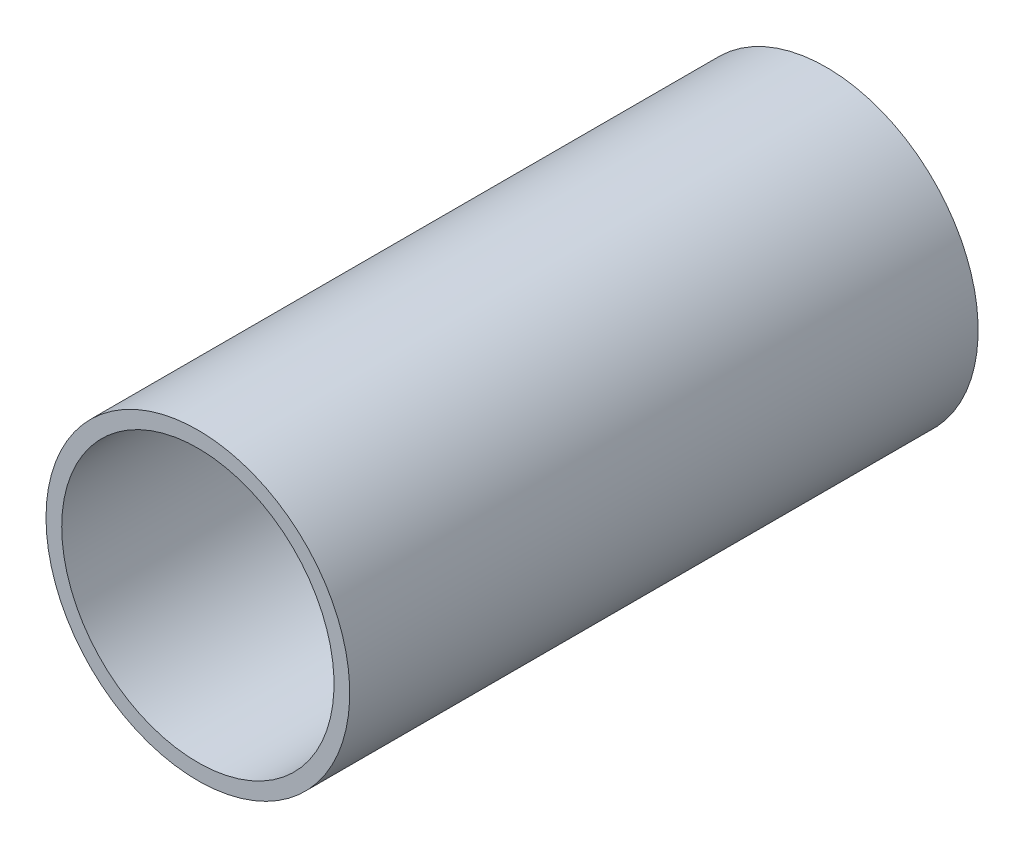
from build123d import *

# Parameters (mm, degrees)
SKETCH1_R           = 3.683
SKETCH1_R_2         = 3.302
BOSS_EXTRUDE1_DEPTH = 15.24
SCALE1_SCALE        = 2


with BuildPart() as part:
    # Sketch1 → Boss-Extrude1 (new body)
    with BuildSketch(Plane.XY):
        with Locations(Location((0, 0, 0), (0, 0, 180))):
            Circle(SKETCH1_R)
        with Locations(Location((0, 0, 0), (0, 0, 180))):
            Circle(SKETCH1_R_2, mode=Mode.SUBTRACT)
    extrude(amount=BOSS_EXTRUDE1_DEPTH)


with BuildPart() as part_1:
    # Scale1: scaled about (0, 0, 0)
    add(part.part.scale(SCALE1_SCALE))


solid = part_1.part
